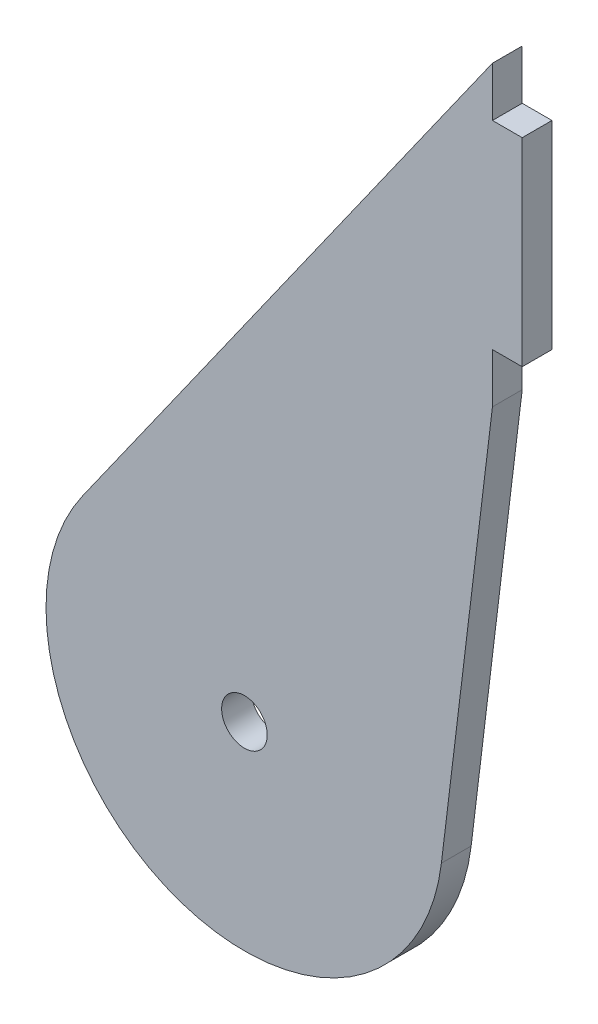
from build123d import *

# Parameters (mm, degrees)
BOSS_EXTRUDE1_DEPTH = 3
SKETCH2_R           = 2.3
CUT_EXTRUDE1_DEPTH  = 10
SKETCH4_W           = 3
SKETCH4_H           = 20
BOSS_EXTRUDE3_DEPTH = 3


with BuildPart() as part:
    # Sketch1 → Boss-Extrude1 (new body)
    with BuildSketch(Plane.XY):
        with BuildLine():
            Line((-16.33027103, 11.546525368), (25, 70))
            Line((25, 70), (25, 40))
            Line((25, 40), (19.854388756, -2.408992972))
            ThreePointArc((19.854388756, -2.408992972), (-7.196803073, -18.660279353), (-16.33027103, 11.546525368))
        make_face()
    extrude(amount=-BOSS_EXTRUDE1_DEPTH)

    # Sketch2 → Cut-Extrude1 (cut)
    with BuildSketch(Plane.XY):
        Circle(SKETCH2_R)
    extrude(amount=-CUT_EXTRUDE1_DEPTH, mode=Mode.SUBTRACT)

    # Sketch4 → Boss-Extrude3 (add)
    with BuildSketch(Plane(origin=(25, 0, 0), x_dir=(0, 0, -1), z_dir=(1, 0, 0))):
        with Locations((1.5, 55)):
            Rectangle(SKETCH4_W, SKETCH4_H)
    extrude(amount=BOSS_EXTRUDE3_DEPTH)


solid = part.part
